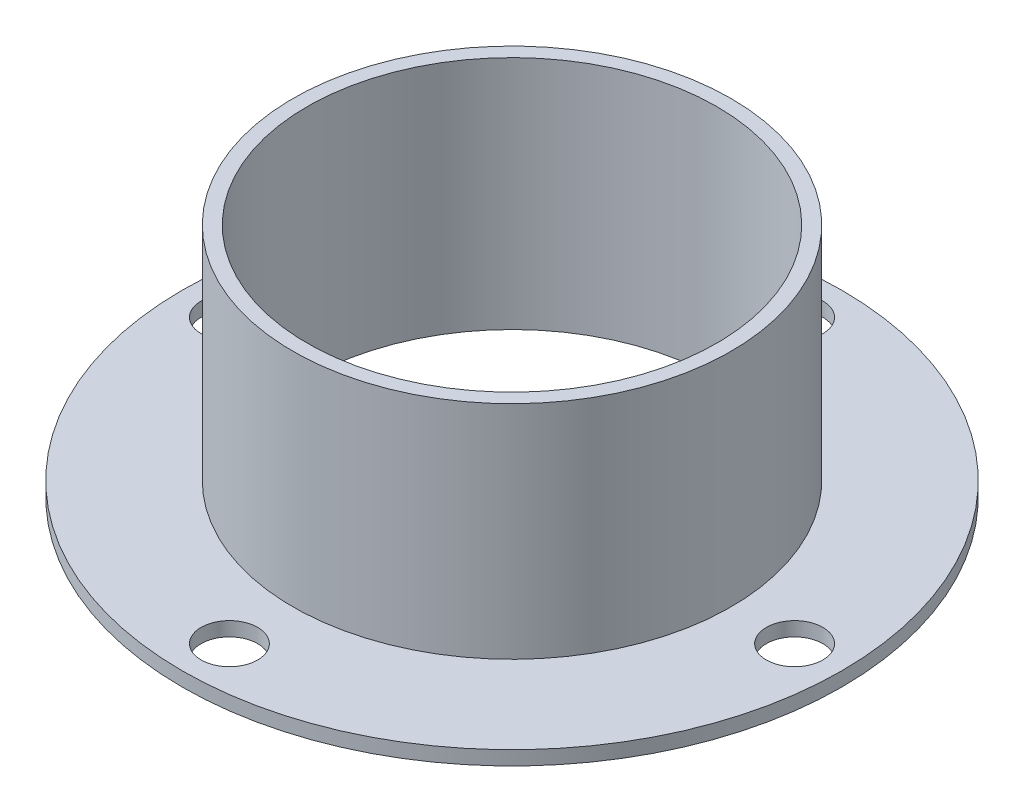
from build123d import *

# Parameters (mm, degrees)
SKETCH_2_R          = 6
CUT_EXTRUDE_1_DEPTH = 110.585582993


with BuildPart() as part:
    # 草图1 → 旋转1 (revolve)
    with BuildSketch(Plane.XY, mode=Mode.PRIVATE) as revolve_1_sk:
        Polygon((43.5, 50), (43.5, 0), (70, 0), (70, 3), (46.5, 3), (46.5, 50), align=None)
    revolve(revolve_1_sk.sketch.rotate(Axis((0, 0, 0), (0, 1, 0)), 90), axis=Axis((0, 0, 0), (0, 1, 0)))

    # 草图2 → 切除-拉伸1 (cut, through all)
    with BuildSketch(Plane(origin=(0, 3, 0), x_dir=(1, 0, 0), z_dir=(0, 1, 0))):
        with Locations(Location((0, 60, 0), (0, 0, 270))):
            Circle(SKETCH_2_R)
        with Locations(Location((60, 0, 0), (0, 0, 270))):
            Circle(SKETCH_2_R)
        with Locations(Location((0, -60, 0), (0, 0, 270))):
            Circle(SKETCH_2_R)
        with Locations(Location((-60, 0, 0), (0, 0, 270))):
            Circle(SKETCH_2_R)
    extrude(amount=-CUT_EXTRUDE_1_DEPTH, mode=Mode.SUBTRACT)


solid = part.part
